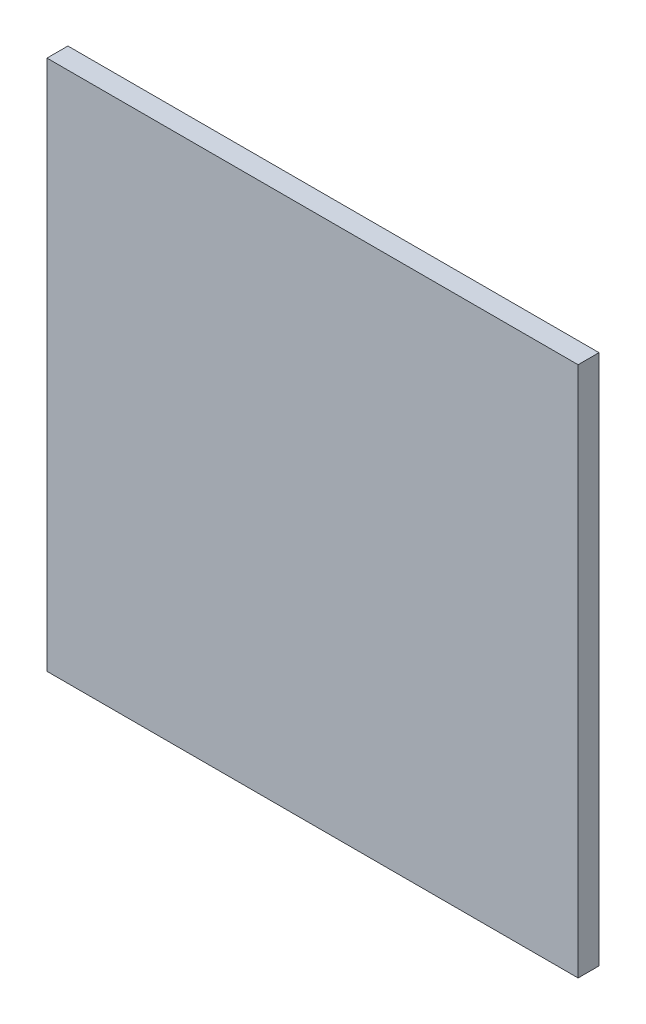
SolidWorks part; units mm, degrees
material "普通碳钢"
ref_plane "Front Plane" through (0, 0, 0) normal (0, 0, 1) x (1, 0, 0)
ref_plane "Top Plane" through (0, 0, 0) normal (0, 1, 0) x (1, 0, 0)
ref_plane "Right Plane" through (0, 0, 0) normal (1, 0, 0) x (0, 0, -1)
sketch "Sketch1" plane through (0, 0, 0) normal (0, 0, 1) x (1, 0, 0)
  line L1 (-127, 127) -> (127, 127)
  line L2 (-127, 127) -> (-127, -127)
  line L3 (-127, -127) -> (127, -127)
  line L4 (127, 127) -> (127, -127)
  dimension "D1" = 254
  dimension "D2" = 127
  dimension "D3" = 254
  dimension "D4" = 127
extrude "Boss-Extrude1" add sketch "Sketch1" along normal mid plane 10
